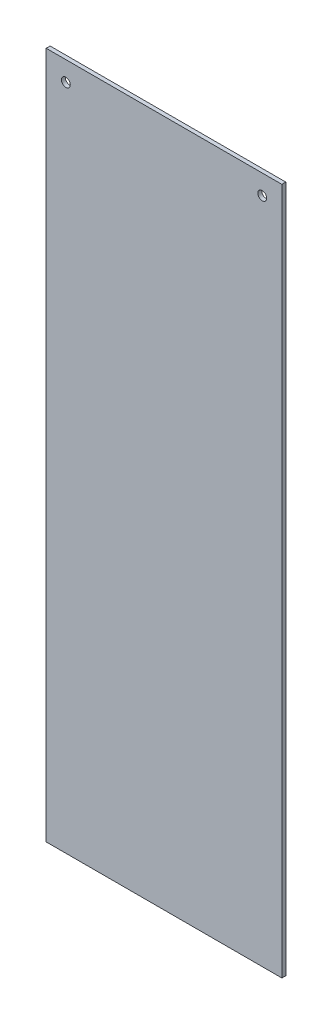
SolidWorks part; units mm, degrees
material "PVC 0.007 塑化"
ref_plane "前视基准面" through (0, 0, 0) normal (0, 0, 1) x (1, 0, 0)
ref_plane "上视基准面" through (0, 0, 0) normal (0, 1, 0) x (1, 0, 0)
ref_plane "右视基准面" through (0, 0, 0) normal (1, 0, 0) x (0, 0, -1)
sketch "草图1" plane through (0, 0, 0) normal (0, 0, 1) x (1, 0, 0)
  line L1 (-60, 175) -> (60, 175)
  line L2 (-60, 175) -> (-60, -175)
  line L3 (-60, -175) -> (60, -175)
  line L4 (60, 175) -> (60, -175)
  line L5 (0, -175) -> (0, 175) construction
  line L6 (-60, 0) -> (60, 0) construction
  point P0 (0, 0)
  dimension "D1" = 120
  dimension "D2" = 350
extrude "凸台-拉伸1" add sketch "草图1" along normal blind 2
sketch "草图2" plane through (0, 0, 2) normal (0, 0, 1) x (1, 0, 0)
  line L0 (0, 175) -> (0, -175) construction
  line L1 (60, 175) -> (-60, 175) construction
  line L2 (-60, -175) -> (60, -175) construction
  line L3 (-50, 165) -> (50, 165) construction
  circle A0 centre (-50, 165) radius 2.25
  circle A1 centre (50, 165) radius 2.25
  dimension "D3" = 4.5
  dimension "D1" = 100
  dimension "D2" = 10
extrude "切除-拉伸1" cut sketch "草图2" against normal blind 10
